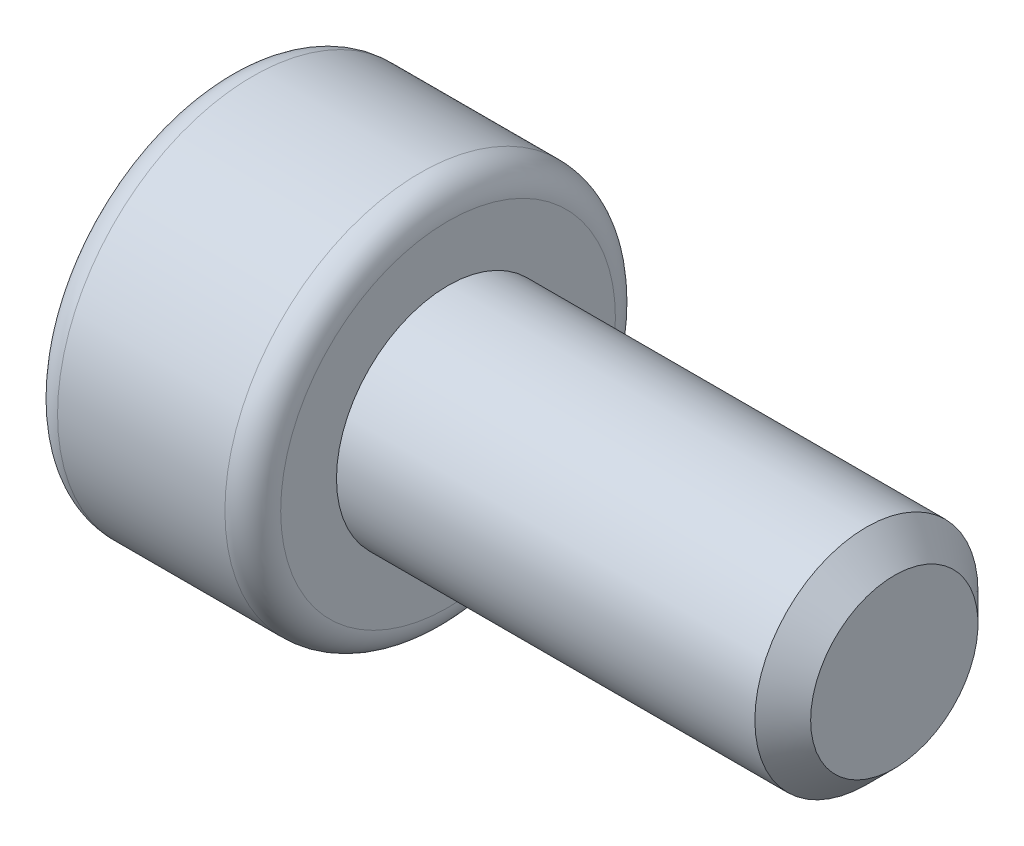
SolidWorks part; units mm, degrees
material "AISI 304"
ref_plane "Front Plane" through (0, 0, 0) normal (0, 0, 1) x (1, 0, 0)
ref_plane "Top Plane" through (0, 0, 0) normal (0, 1, 0) x (1, 0, 0)
ref_plane "Right Plane" through (0, 0, 0) normal (1, 0, 0) x (0, 0, -1)
sketch "Sketch1" plane through (0, 0, 0) normal (0, 0, 1) x (1, 0, 0)
  line L0 (-4.7092, 0) -> (12, 0) construction
  line L1 (0, 0) -> (0, 3.5)
  line L2 (0, 3.5) -> (4, 3.5)
  line L3 (4, 3.5) -> (4, 2)
  line L4 (4, 2) -> (12, 2)
  line L5 (12, 2) -> (12, 0)
  line L6 (12, 0) -> (0, 0)
  dimension "D1" = 7
  dimension "D2" = 4
  dimension "D3" = 4
  dimension "D4" = 8
revolve "Revolve1" add sketch "Sketch1" angle 360 about L0
cosmetic thread "Cosmetic Thread1" parameters "D2"=3
sketch "Sketch4" plane through (0, 0, 0) normal (-1, 0, 0) x (0, 0, 1)
  line L1 (-1.7321, 0) -> (-0.866, -1.5)
  line L2 (-0.866, -1.5) -> (0.866, -1.5)
  line L3 (0.866, -1.5) -> (1.7321, 0)
  line L4 (1.7321, 0) -> (0.866, 1.5)
  line L5 (0.866, 1.5) -> (-0.866, 1.5)
  line L6 (-0.866, 1.5) -> (-1.7321, 0)
  circle A0 centre (0, 0) radius 1.5 construction
extrude "Cut-Extrude1" cut sketch "Sketch4" against normal blind 2
fillet "Fillet1" radius 0.5 2 edges at (4, 0, 3.5) (0, 0, 3.5)
chamfer "Chamfer1" distance 0.1 angle 80 6 edges at (0, -0.75, -1.299) (0, -1.5, 0) (0, -0.75, 1.299) (0, 0.75, 1.299) (0, 1.5, 0) (0, 0.75, -1.299)
chamfer "Chamfer2" distance 0.5 angle 45 1 edges at (12, 0, 2)
